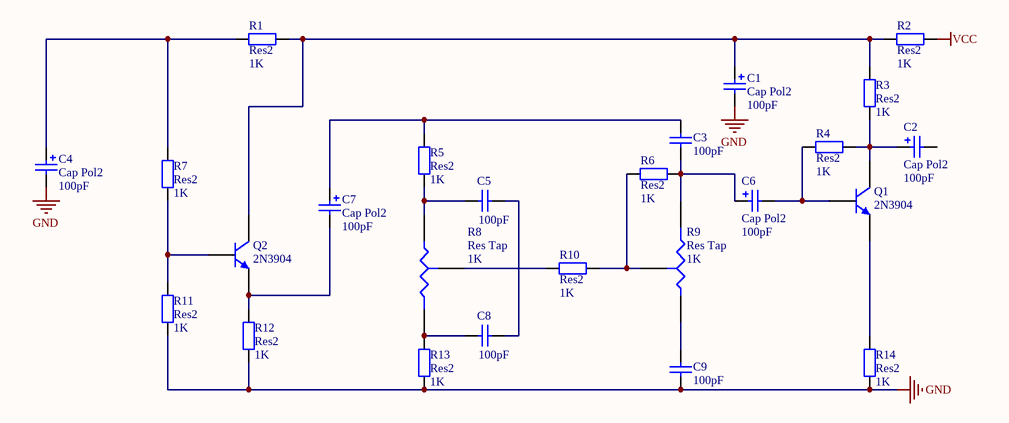
[diagram p0: MISC80684-7.SchDoc]
# Altium project MISC80684-2.PrjPcb
4 sheets, 64 parts. Net scope: flat (ports and power ports of the same name join across sheets).
Board files: MISC80684.PcbDoc, MISC80684-4.PcbDoc, MISC80684-5.PcbDoc, MISC80684-6.PcbDoc
Sheets:
  MISC80684-7.SchDoc
  MISC80684-8.SchDoc
  MISC80684-9.SchDoc
  MISC80684-10.SchDoc

## Sheet MISC80684-7.SchDoc
size A4

### Parts
C1  Cap Pol2  value 100pF  [POLAR0.8]
C2  Cap Pol2  value 100pF  [POLAR0.8]
C3  value 100pF  [RAD-0.3]  (hidden comment: Cap)
C4  Cap Pol2  value 100pF  [POLAR0.8]
C5  value 100pF  [RAD-0.3]  (hidden comment: Cap)
C6  Cap Pol2  value 100pF  [POLAR0.8]
C7  Cap Pol2  value 100pF  [POLAR0.8]
C8  value 100pF  [RAD-0.3]  (hidden comment: Cap)
C9  value 100pF  [RAD-0.3]  (hidden comment: Cap)
Q1  2N3904  [TO-92A]
Q2  2N3904  [TO-92A]
R1  Res2  value 1K  [AXIAL-0.4]
R2  Res2  value 1K  [AXIAL-0.4]
R3  Res2  value 1K  [AXIAL-0.4]
R4  Res2  value 1K  [AXIAL-0.4]
R5  Res2  value 1K  [AXIAL-0.4]
R6  Res2  value 1K  [AXIAL-0.4]
R7  Res2  value 1K  [AXIAL-0.4]
R8  Res Tap  value 1K  [VR3]
R9  Res Tap  value 1K  [VR3]
R10  Res2  value 1K  [AXIAL-0.4]
R11  Res2  value 1K  [AXIAL-0.4]
R12  Res2  value 1K  [AXIAL-0.4]
R13  Res2  value 1K  [AXIAL-0.4]
R14  Res2  value 1K  [AXIAL-0.4]

### Nets
GND: C1.2 C4.2 C9.1 R11.1 R12.1 R13.1 R14.1
VCC: R2.2
NetC1_1: C1.1 Q2.3(C) R1.1 R2.1 R3.1
NetC2_1: C2.1 Q1.3(C) R3.2 R4.1
NetC3_1: C3.1 C6.1 R6.1 R9.2(B)
NetC3_2: C3.2 C7.1 R5.2
NetC4_1: C4.1 R1.2 R7.2
NetC5_1: C5.1 R5.1 R8.1(A)
NetC5_2: C5.2 C8.2
NetC6_2: C6.2 Q1.2(B) R4.2
NetC7_2: C7.2 Q2.1(E) R12.2
NetC8_1: C8.1 R8.2(B) R13.2
NetC9_2: C9.2 R9.1(A)
NetQ1_1: Q1.1(E) R14.2
NetQ2_2: Q2.2(B) R7.1 R11.2
NetR6_2: R6.2 R9.3(TAP) R10.1
NetR8_3: R8.3(TAP) R10.2

Not connected (* = marked no-connect by the designer): C2 2

### Library data of the parts
C1 C2 C4 C6 C7 = Cap Pol2: Polarized Capacitor (Axial); Published: 8-Jun-2000; LatestRevisionDate: 17-Jul-2002; LatestRevisionNote: Re-released for DXP Platform.; PackageReference: POLAR0.8; PackageDescription: Polarized Capacitor; 2 Leads; Publisher: Altium Limited
C3 C5 C8 C9 = Cap: Capacitor; Published: 8-Jun-2000; LatestRevisionDate: 17-Jul-2002; LatestRevisionNote: Re-released for DXP Platform.; PackageReference: RAD-0.3; PackageDescription: Radial Cap, Thru-Hole; 2 Leads; 0.3 in Pin Spacing; Publisher: Altium Limited
Q1 Q2 = 2N3904: NPN General Purpose Amplifier; Published: 8-Jun-2000; LatestRevisionDate: 15-Jan-2003; LatestRevisionNote: PCB Footprint 'BCY-W3/D4.7' replaced; DatasheetVersion: 1997; PackageVersion: Sep-1998; PackageReference: TO-92A; PackageDescription: TO, Flat Index; 3 In-Line, Axial Leads; Body Dia. 4.5mm; Leads 0.51 x 0.48 mm (max); ComponentLink1Description: Manufacturer Link; ComponentLink2Description: Datasheet; ComponentLink2URL: http://www.fairchildsemi.com/ds/2N%2F2N3904.pdf; Publisher: Altium Limited
R1-R7 R10-R14 = Res2: Resistor; Published: 8-Jun-2000; LatestRevisionDate: 17-Jul-2002; LatestRevisionNote: Re-released for DXP Platform.; PackageReference: AXIAL-0.4; PackageDescription: Axial Device, Thru-Hole; 2 Leads; 0.4 in Pin Spacing; Publisher: Altium Limited
R8 R9 = Res Tap: Tapped Resistor; Sim Note: Enter the Resistance value and the set point into parameter fields.; Set Position: 0.5; Published: 24-Mar-1999; LatestRevisionDate: 17-Jul-2002; LatestRevisionNote: Re-released for DXP Platform.; PackageReference: VR3; PackageDescription: Variable Resistor, Thru-Hole; 3 Leads; Publisher: Altium Limited

## Sheet MISC80684-8.SchDoc
size A4
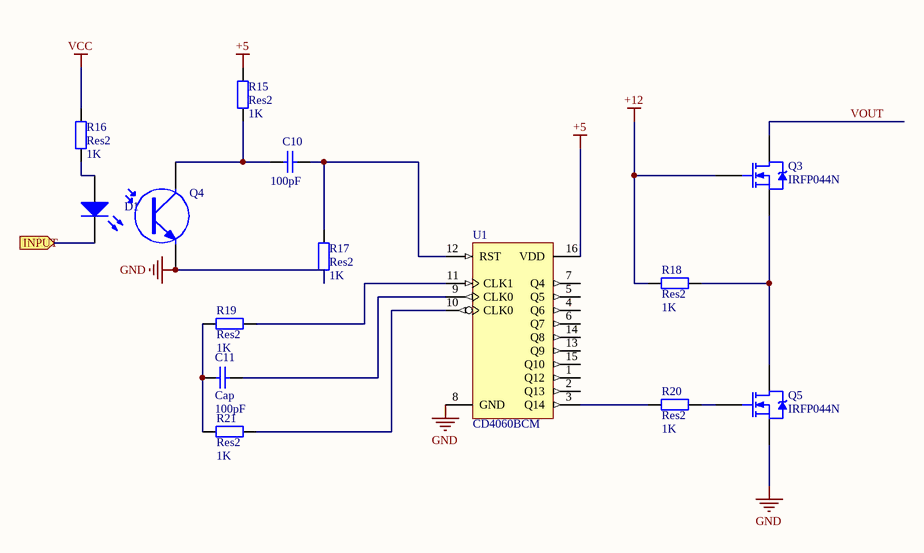
[diagram p1: MISC80684-8.SchDoc]

### Parts
C10  value 100pF  [RAD-0.3]  (hidden comment: Cap)
C11  Cap  value 100pF  [RAD-0.3]
D1  LED0  [LED-0]  (value not drawn)
Q3  IRFP044N  [TO-247AC]
Q4  Photo NPN  [TO-220_A]  (value not drawn)
Q5  IRFP044N  [TO-247AC]
R15  Res2  value 1K  [AXIAL-0.4]
R16  Res2  value 1K  [AXIAL-0.4]
R17  Res2  value 1K  [AXIAL-0.4]
R18  Res2  value 1K  [AXIAL-0.4]
R19  Res2  value 1K  [AXIAL-0.4]
R20  Res2  value 1K  [AXIAL-0.4]
R21  Res2  value 1K  [AXIAL-0.4]
U1  CD4060BCM  [M16A_N]

### Ports
INPUT (in)

### Nets
+5: R15.1 U1.16(VDD)  [project net L]
+12: Q3.1(G) R18.2
GND: Q4.3(E) Q5.3(S) R17.1 U1.8(GND)
VCC: R16.1
VOUT: Q3.2(D)
NetC10_1: C10.1 Q4.1(C) R15.2
NetC10_2: C10.2 R17.2 U1.12(RST)
NetC11_1: C11.1 R19.2 R21.2
NetC11_2: C11.2 U1.9(CLK0)
NetD1_1: D1.1(A) R16.2
NetD1_2: D1.2(K) ; port INPUT
NetQ3_3: Q3.3(S) Q5.2(D) R18.1
NetQ5_1: Q5.1(G) R20.1
NetR19_1: R19.1 U1.11(CLK1)
NetR20_2: R20.2 U1.3(Q14)
NetR21_1: R21.1 U1.10(CLK0)

Not connected (* = marked no-connect by the designer): U1 1(Q12) 2(Q13) 4(Q6) 5(Q5) 6(Q7) 7(Q4) 13(Q9) 14(Q8) 15(Q10)

### Library data of the parts
C10 C11 = Cap: Capacitor; Published: 8-Jun-2000; LatestRevisionDate: 17-Jul-2002; LatestRevisionNote: Re-released for DXP Platform.; PackageReference: RAD-0.3; PackageDescription: Radial Cap, Thru-Hole; 2 Leads; 0.3 in Pin Spacing; Publisher: Altium Limited
D1 = LED0: Typical INFRARED GaAs LED; Published: 8-Jun-2000; LatestRevisionDate: 08-Jul-2005; LatestRevisionNote: Mech Layer 1 removed.; PackageReference: LED-0; PackageDescription: LED; 2 Leads; Publisher: Altium Limited
Q3 Q5 = IRFP044N: HEXFET Power MOSFET; Note: Pin 2 is electrically connected to the Heatsink (4).; Published: 8-Jun-2000; LatestRevisionDate: 17-Jul-2002; LatestRevisionNote: Re-released for DXP Platform.; DatasheetVersion: Aug-1997; PackageVersion: Aug-1997; PackageReference: TO-247AC; PackageDescription: SIP with Mounting Hole; 3 Leads; Body 20 x 15.6 x 5 mm (typ); Pitch 5.45 mm; Code_JEDEC: TO-247-AC; ComponentLink1Description: Manufacturer Link; ComponentLink2Description: Datasheet; ComponentLink2URL: http://www.irf.com/product-info/datasheets/data/irfp044n.pdf; Publisher: Altium Limited
Q4 = Photo NPN: NPN Phototransistor; Published: 24-Mar-1999; LatestRevisionDate: 17-Jul-2002; LatestRevisionNote: Re-released for DXP Platform.; PackageReference: TO-220_A; Code_JEDEC: TO-220-AC; Publisher: Altium Limited
R15-R21 = Res2: Resistor; Published: 8-Jun-2000; LatestRevisionDate: 17-Jul-2002; LatestRevisionNote: Re-released for DXP Platform.; PackageReference: AXIAL-0.4; PackageDescription: Axial Device, Thru-Hole; 2 Leads; 0.4 in Pin Spacing; Publisher: Altium Limited
U1 = CD4060BCM: 14-Stage Ripple Carry Binary Counter; Published: 17-Jul-2002; LatestRevisionDate: 13-Apr-2006; LatestRevisionNote: IPC-7351 Footprint Added.; DatasheetVersion: Jan-1999; PackageVersion: 2000; PackageReference: M16A; PackageDescription: 16-Pin Small Outline Integrated Circuit 1.27 mm Pitch; Code_IPC: SOIC127P600-16; ComponentLink1Description: Manufacturer Link; ComponentLink2Description: Datasheet; ComponentLink2URL: http://www.fairchildsemi.com/ds/CD%2FCD4040BC.pdf; Publisher: Altium Limited

## Sheet MISC80684-9.SchDoc
size A4
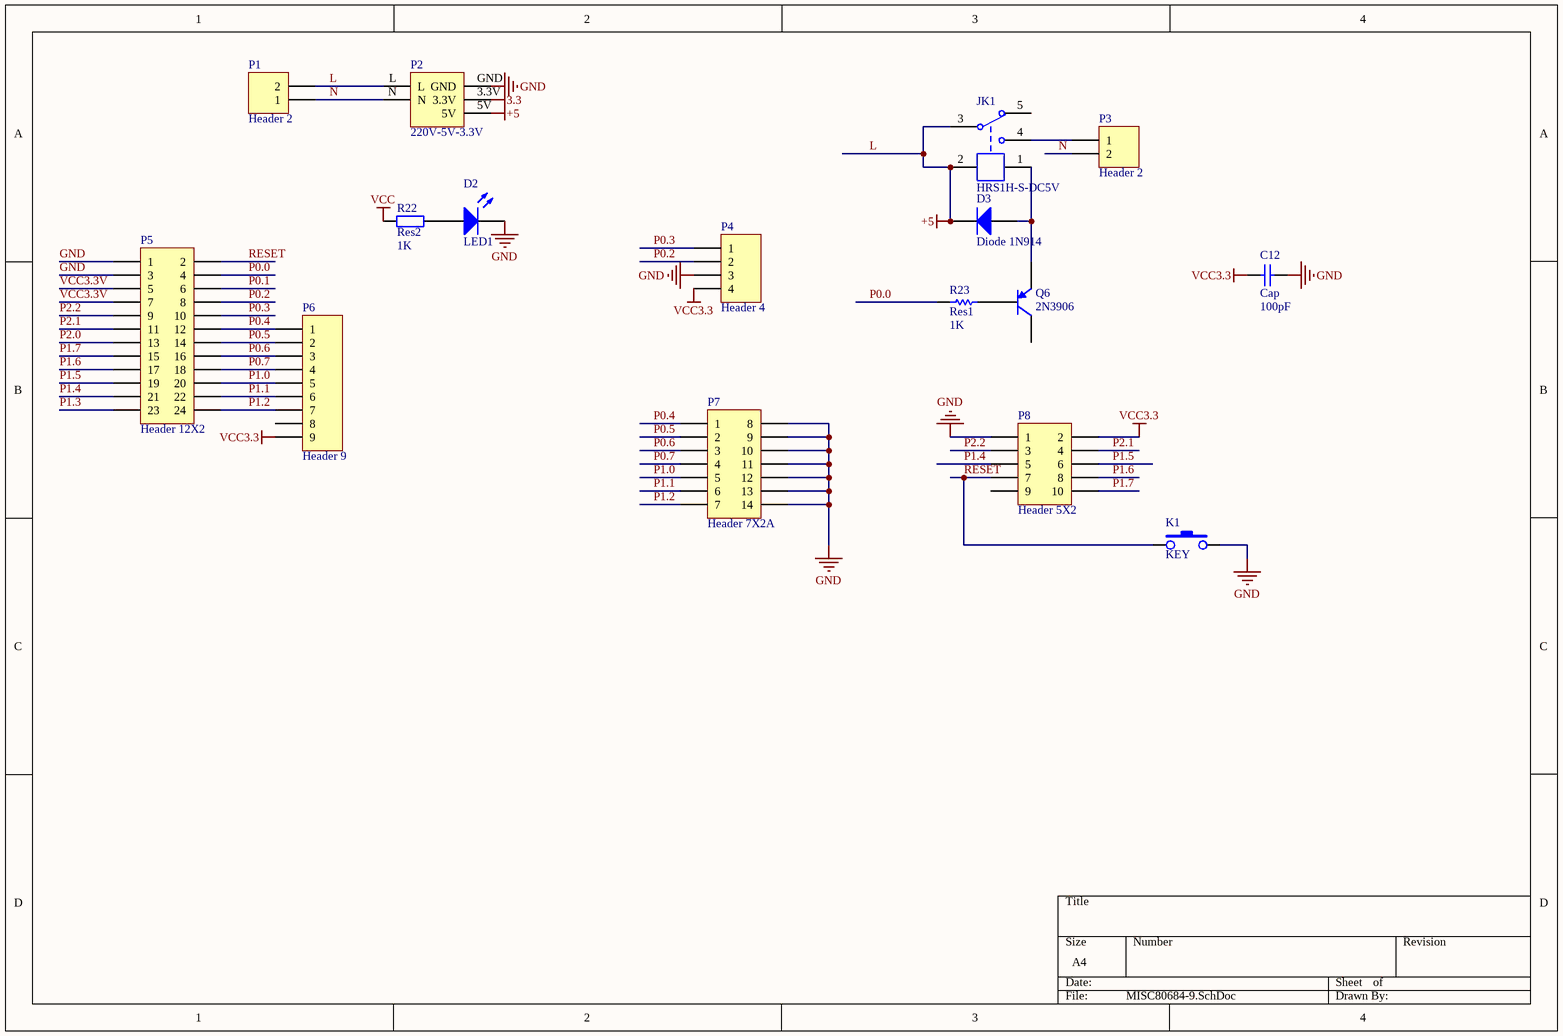
[diagram p2: MISC80684-9.SchDoc]

### Parts
C12  Cap  value 100pF  [RAD-0.3]
D2  LED1  [LED-1]
D3  Diode 1N914  [DO-35]
JK1  HRS1H-S-DC5V  [HRS1H]
K1  KEY  [DIP-3X6X4.3]
P1  Header 2  [HDR1X2]
P2  220V-5V-3.3V  [HDR2X3]
P3  Header 2  [HDR1X2]
P4  Header 4  [HDR1X4]
P5  Header 12X2  [HDR2X12]
P6  Header 9  [HDR1X9]
P7  Header 7X2A  [HDR2X7_CEN]
P8  Header 5X2  [HDR2X5]
Q6  2N3906  [TO-92A]
R22  Res2  value 1K  [AXIAL-0.4]
R23  Res1  value 1K  [AXIAL-0.3]

### Nets
3.3: P2.3.3V
GND: C12.2 D2.2(K) K1.3 P2.GND P4.3 P5.1 P5.3 P7.8 P7.9 P7.10 P7.11 P7.12 P7.13 P7.14 P8.1
L: D3.2(K) JK1.2 JK1.3 P1.2 P2.5V P2.L  [also labelled +5]
VCC: R22.1
VCC3.3: C12.1 P4.4 P6.9 P8.2
N: P1.1 P2.N P3.2
P0.0: P5.4 R23.1
P0.1: P5.6
P0.2: P4.2 P5.8
P0.3: P4.1 P5.10
P0.4: P5.12 P6.1 P7.1
P0.5: P5.14 P6.2 P7.2
P0.6: P5.16 P6.3 P7.3
P0.7: P5.18 P6.4 P7.4
P1.0: P5.20 P6.5 P7.5
P1.1: P5.22 P6.6 P7.6
P1.2: P5.24 P6.7 P7.7
P1.3: P5.23
P1.4: P5.21 P8.5
P1.5: P5.19 P8.6
P1.6: P5.17 P8.8
P1.7: P5.15 P8.10
P2.0: P5.13
P2.1: P5.11 P8.4
P2.2: P5.9 P8.3
RESET: K1.1 P5.2 P8.7
VCC3.3V: P5.5 P5.7
NetD2_1: D2.1(A) R22.2
NetD3_1: D3.1(A) JK1.1 Q6.1(E)
NetJK1_4: JK1.4 P3.1
NetQ6_2: Q6.2(B) R23.2

Not connected (* = marked no-connect by the designer): JK1 5; P6 8; P8 9; Q6 3(C)

### Library data of the parts
C12 = Cap: Capacitor; Published: 8-Jun-2000; LatestRevisionDate: 17-Jul-2002; LatestRevisionNote: Re-released for DXP Platform.; PackageReference: RAD-0.3; PackageDescription: Radial Cap, Thru-Hole; 2 Leads; 0.3 in Pin Spacing; Publisher: Altium Limited
D2 = LED1: Typical RED GaAs LED; Published: 8-Jun-2000; LatestRevisionDate: 08-Jul-2005; LatestRevisionNote: Mech Layer 1 removed.; PackageReference: LED-1; PackageDescription: LED; 2 Leads; Publisher: Altium Limited
D3 = Diode 1N914: High Conductance Fast Diode; Published: 8-Jun-2000; LatestRevisionDate: 17-Jul-2002; LatestRevisionNote: Re-released for DXP Platform.; DatasheetVersion: 1997; PackageReference: DO-35; PackageDescription: Diode, Axial; Body 3.8 x 1.9 mm (LxDia. max), Lead Dia. 0.53 mm (max); Code_JEDEC: DO-204-AH; ComponentLink1Description: Manufacturer Link; ComponentLink2Description: Datasheet; ComponentLink2URL: http://www.fairchildsemi.com/ds/1N%2F1N4448.pdf; Publisher: Altium Limited
JK1 = HRS1H-S-DC5V: 5V一组转换
P1 P3 = Header 2: Header, 2-Pin; LatestRevisionDate: 17-Jul-2002; LatestRevisionNote: Re-released for DXP Platform.; Publisher: Altium Limited
P2 = Header 3X2: Header, 3-Pin, Dual row; LatestRevisionDate: 17-Jul-2002; LatestRevisionNote: Re-released for DXP Platform.; Publisher: Altium Limited
P4 = Header 4: Header, 4-Pin; LatestRevisionDate: 17-Jul-2002; LatestRevisionNote: Re-released for DXP Platform.; Publisher: Altium Limited
P5 = Header 12X2: Header, 12-Pin, Dual row; LatestRevisionDate: 17-Jul-2002; LatestRevisionNote: Re-released for DXP Platform.; Publisher: Altium Limited
P6 = Header 9: Header, 9-Pin; LatestRevisionDate: 17-Jul-2002; LatestRevisionNote: Re-released for DXP Platform.; Publisher: Altium Limited
P7 = Header 7X2A: Header, 7-Pin, Dual row; LatestRevisionDate: 17-Jul-2002; LatestRevisionNote: Re-released for DXP Platform.; Publisher: Altium Limited
P8 = Header 5X2: Header, 5-Pin, Dual row; LatestRevisionDate: 17-Jul-2002; LatestRevisionNote: Re-released for DXP Platform.; Publisher: Altium Limited
Q6 = 2N3906: PNP General Purpose Amplifier; Published: 8-Jun-2000; LatestRevisionDate: 15-Jan-2003; LatestRevisionNote: PCB Footprint 'BCY-W3/D4.7' replaced; DatasheetVersion: 1997; PackageVersion: Sep-1998; PackageReference: TO-92A; PackageDescription: TO, Flat Index; 3 In-Line, Axial Leads; Body Dia. 4.5mm; Leads 0.51 x 0.48 mm (max); ComponentLink1Description: Manufacturer Link; ComponentLink2Description: Datasheet; ComponentLink2URL: http://www.fairchildsemi.com/ds/2N%2F2N3906.pdf; Publisher: Altium Limited
R22 = Res2: Resistor; Published: 8-Jun-2000; LatestRevisionDate: 17-Jul-2002; LatestRevisionNote: Re-released for DXP Platform.; PackageReference: AXIAL-0.4; PackageDescription: Axial Device, Thru-Hole; 2 Leads; 0.4 in Pin Spacing; Publisher: Altium Limited
R23 = Res1: Resistor; Published: 8-Jun-2000; LatestRevisionDate: 17-Jul-2002; LatestRevisionNote: Re-released for DXP Platform.; PackageReference: AXIAL-0.3; PackageDescription: Axial Device, Thru-Hole; 2 Leads; 0.3 in Pin Spacing; Publisher: Altium Limited

## Sheet MISC80684-10.SchDoc
size A4
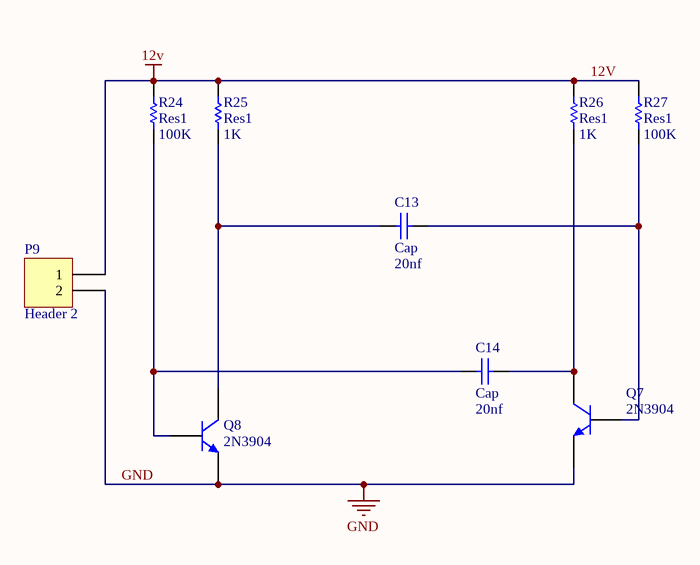
[diagram p3: MISC80684-10.SchDoc]

### Parts
C13  Cap  value 20nf  [RAD-0.3]
C14  Cap  value 20nf  [RAD-0.3]
P9  Header 2  [HDR1X2]
Q7  2N3904  [TO-92A]
Q8  2N3904  [TO-92A]
R24  Res1  value 100K  [AXIAL-0.3]
R25  Res1  value 1K  [AXIAL-0.3]
R26  Res1  value 1K  [AXIAL-0.3]
R27  Res1  value 100K  [AXIAL-0.3]

### Nets
12V: P9.1 R24.2 R25.2 R26.2 R27.2
GND: P9.2 Q7.1(E) Q8.1(E)
NetC13_1: C13.1 Q8.3(C) R25.1
NetC13_2: C13.2 Q7.2(B) R27.1
NetC14_1: C14.1 Q8.2(B) R24.1
NetC14_2: C14.2 Q7.3(C) R26.1

### Library data of the parts
C13 C14 = Cap: Capacitor; Published: 8-Jun-2000; LatestRevisionDate: 17-Jul-2002; LatestRevisionNote: Re-released for DXP Platform.; PackageReference: RAD-0.3; PackageDescription: Radial Cap, Thru-Hole; 2 Leads; 0.3 in Pin Spacing; Publisher: Altium Limited
P9 = Header 2: Header, 2-Pin; LatestRevisionDate: 17-Jul-2002; LatestRevisionNote: Re-released for DXP Platform.; Publisher: Altium Limited
Q7 Q8 = 2N3904: NPN General Purpose Amplifier; Published: 8-Jun-2000; LatestRevisionDate: 15-Jan-2003; LatestRevisionNote: PCB Footprint 'BCY-W3/D4.7' replaced; DatasheetVersion: 1997; PackageVersion: Sep-1998; PackageReference: TO-92A; PackageDescription: TO, Flat Index; 3 In-Line, Axial Leads; Body Dia. 4.5mm; Leads 0.51 x 0.48 mm (max); ComponentLink1Description: Manufacturer Link; ComponentLink2Description: Datasheet; ComponentLink2URL: http://www.fairchildsemi.com/ds/2N%2F2N3904.pdf; Publisher: Altium Limited
R24-R27 = Res1: Resistor; Published: 8-Jun-2000; LatestRevisionDate: 17-Jul-2002; LatestRevisionNote: Re-released for DXP Platform.; PackageReference: AXIAL-0.3; PackageDescription: Axial Device, Thru-Hole; 2 Leads; 0.3 in Pin Spacing; Publisher: Altium Limited

## Nets that join several sheets
GND: MISC80684-7 (7 pins), MISC80684-8 (Q4.3 Q5.3 R17.1 U1.8), MISC80684-9 (15 pins), MISC80684-10 (P9.2 Q7.1 Q8.1)
L: MISC80684-8 (R15.1 U1.16), MISC80684-9 (6 pins)
VCC: MISC80684-7 (R2.2), MISC80684-8 (R16.1), MISC80684-9 (R22.1)